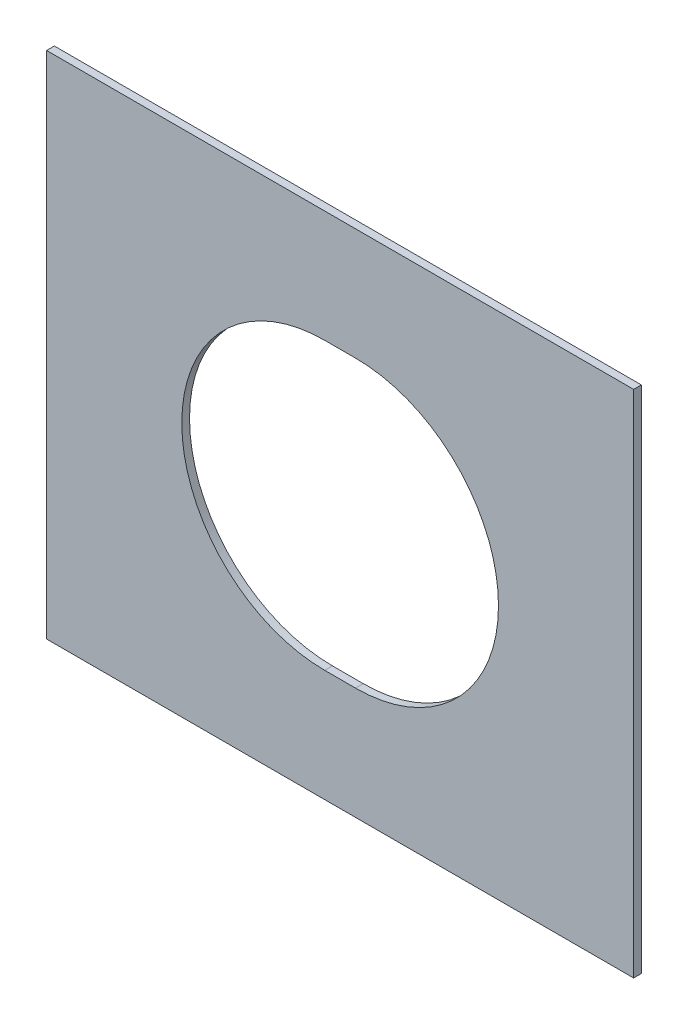
SolidWorks part; units mm, degrees
ref_plane "前视基准面" through (0, 0, 0) normal (0, 0, 1) x (1, 0, 0)
ref_plane "上视基准面" through (0, 0, 0) normal (0, 1, 0) x (1, 0, 0)
ref_plane "右视基准面" through (0, 0, 0) normal (1, 0, 0) x (0, 0, -1)
sketch "草图1" plane through (0, 0, 0) normal (0, 0, 1) x (1, 0, 0)
  line L0 (0, 0) -> (380, 0)
  line L1 (380, 0) -> (380, 330)
  line L2 (380, 330) -> (0, 330)
  line L3 (0, 330) -> (0, 0)
extrude "凸台-拉伸1" add sketch "草图1" along normal blind 5
sketch "草图2" plane through (0, 0, 0) normal (0, 0, -1) x (-1, 0, 0)
  line L1 (-190, 165) -> (-210, 165)
  line L2 (-190, 165) -> (-170, 165)
  line L3 (-210, 72.5) -> (-170, 72.5)
  line L4 (-210, 257.5) -> (-170, 257.5)
  arc A0 (-210, 257.5) -> (-210, 72.5) centre (-210, 165) ccw
  arc A2 (-170, 72.5) -> (-170, 257.5) centre (-170, 165) ccw
extrude "切除-拉伸1" cut sketch "草图2" against normal blind 10
sketch "草图3" plane through (0, 0, 0) normal (0, 0, -1) x (-1, 0, 0)
  line L6 (-210, 72.5) -> (-170, 72.5)
  line L7 (-210, 72.5) -> (-170, 72.5)
  line L8 (-210, 72.5) -> (-200, 72.5)
  line L9 (-210, 257.5) -> (-170, 257.5)
  line L10 (-210, 257.5) -> (-170, 257.5)
  line L11 (-170, 72.5) -> (-180, 72.5)
  arc A0 (-180, 72.5) -> (-180, 257.5) centre (-180, 165) ccw
  arc A2 (-210, 257.5) -> (-210, 72.5) centre (-210, 165) ccw
  arc A3 (-210, 257.5) -> (-210, 72.5) centre (-210, 165) ccw
  arc A4 (-210, 257.5) -> (-210, 72.5) centre (-210, 165) ccw
  arc A5 (-170, 72.5) -> (-170, 257.5) centre (-170, 165) ccw
  arc A6 (-170, 72.5) -> (-170, 257.5) centre (-170, 165) ccw
  arc A7 (-200, 257.5) -> (-200, 72.5) centre (-200, 165) ccw
  arc M5 (-170, 257.5) -> (-170, 72.5) centre (-170, 165) cw
  line M6 (-170, 72.5) -> (-210, 72.5)
  arc M7 (-210, 72.5) -> (-210, 257.5) centre (-210, 165) cw
  line M8 (-210, 257.5) -> (-170, 257.5)
  dimension "D1" = 0
  dimension "D2" = 0
  dimension "D3" = 0
  dimension "D4" = 0
  dimension "D5" = 0
extrude "凸台-拉伸2" add sketch "草图3" against normal blind 5 contours A7 L7 M8 M7 | A0 L10 M6 M5
